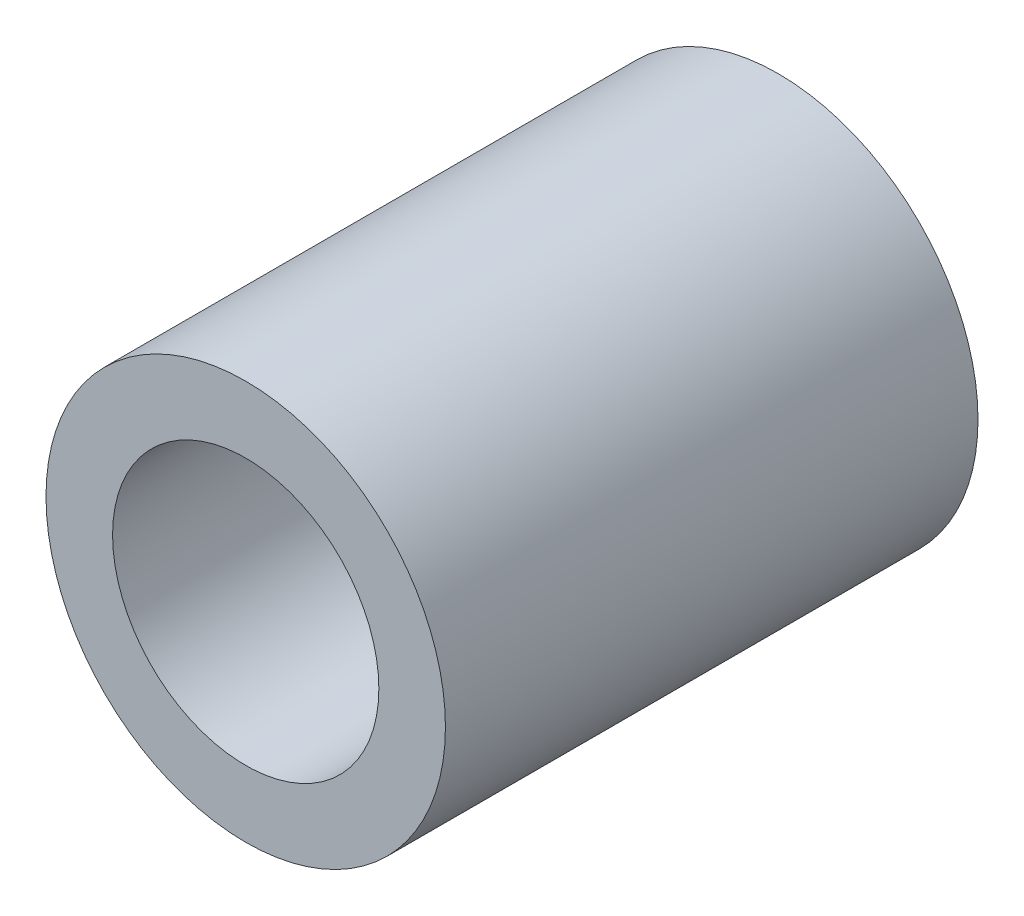
SolidWorks part; units mm, degrees
material "国产6061 "
ref_plane "Front Plane" through (0, 0, 0) normal (0, 0, 1) x (1, 0, 0)
ref_plane "Top Plane" through (0, 0, 0) normal (0, 1, 0) x (1, 0, 0)
ref_plane "Right Plane" through (0, 0, 0) normal (1, 0, 0) x (0, 0, -1)
sketch "Sketch2" plane through (0, 0, 0) normal (0, 0, 1) x (1, 0, 0)
  circle A0 centre (0, 0) radius 7.5
  circle A1 centre (0, 0) radius 5
  dimension "D1" = 10
  dimension "D2" = 15
extrude "Boss-Extrude1" add sketch "Sketch2" along normal mid plane 20
